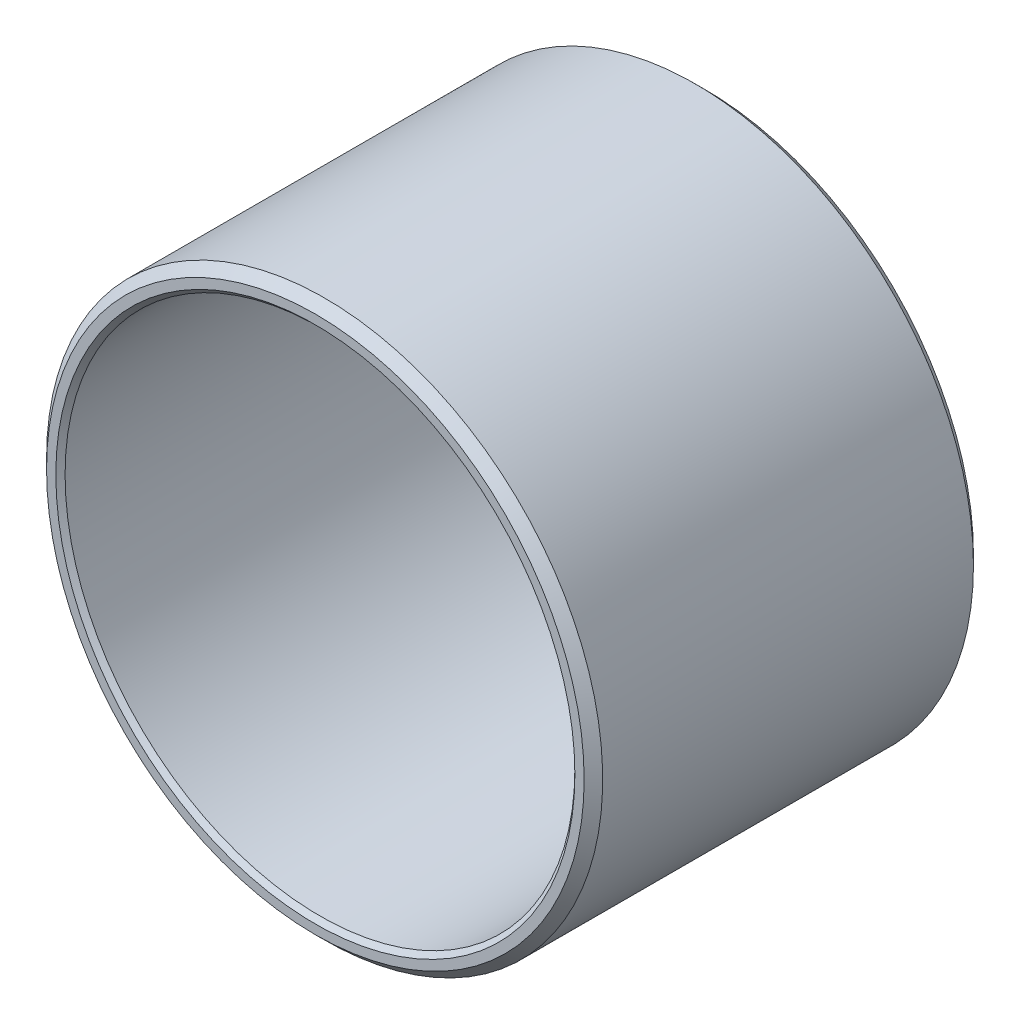
from build123d import *

# Parameters (mm, degrees)
SKETCH1_R           = 60
SKETCH1_R_2         = 55
BOSS_EXTRUDE1_DEPTH = 42
CHAMFER1_SIZE       = 2
CHAMFER2_SIZE       = 1


with BuildPart() as part:
    # Sketch1 → Boss-Extrude1 (new, symmetric)
    with BuildSketch(Plane.XY):
        with Locations(Location((0, 0, 0), (0, 0, 180))):
            Circle(SKETCH1_R)
        with Locations(Location((0, 0, 0), (0, 0, 180))):
            Circle(SKETCH1_R_2, mode=Mode.SUBTRACT)
    extrude(amount=BOSS_EXTRUDE1_DEPTH, both=True)

    # Chamfer1
    chamfer1_edges = [part.edges().sort_by_distance(p)[0] for p in [
        (60, 0, -42),
        (60, 0, 42),
    ]]
    chamfer(chamfer1_edges, length=CHAMFER1_SIZE)

    # Chamfer2
    chamfer2_edges = [part.edges().sort_by_distance(p)[0] for p in [
        (55, 0, -42),
        (55, 0, 42),
    ]]
    chamfer(chamfer2_edges, length=CHAMFER2_SIZE)


solid = part.part
